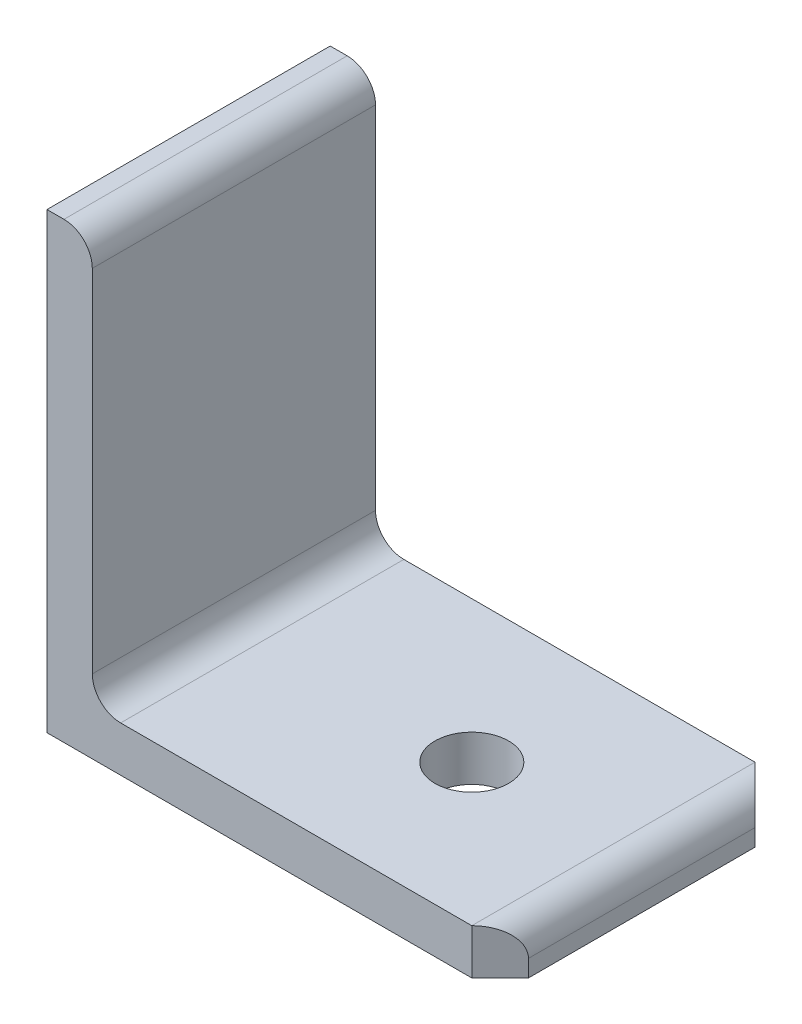
from build123d import *

# Parameters (mm, degrees)
EXTRUDE_1_DEPTH     = 50
SKETCH_2_R          = 6.5
CUT_EXTRUDE_1_DEPTH = 50
FILLET_1_R          = 5
FILLET_2_R          = 5
CHAMFER_1_SIZE      = 5
FILLET_3_R          = 5


with BuildPart() as part:
    # 草图1 → 凸台-拉伸1 (new body)
    with BuildSketch(Plane.XY):
        Polygon((0, 0), (0, -80), (80, -80), (80, -72), (8, -72), (8, 0), align=None)
    extrude(amount=EXTRUDE_1_DEPTH)

    # 草图2 → 切除-拉伸1 (cut)
    with BuildSketch(Plane(origin=(0, -72, 0), x_dir=(1, 0, 0), z_dir=(0, 1, 0))):
        with Locations(Location((50, -25, 0), (0, 0, 270))):
            Circle(SKETCH_2_R)
    extrude(amount=-CUT_EXTRUDE_1_DEPTH, mode=Mode.SUBTRACT)

    # 圆角1
    fillet_1_edges = [part.edges().sort_by_distance(p)[0] for p in [
        (8, -72, 25),
    ]]
    fillet(fillet_1_edges, radius=FILLET_1_R)

    # 圆角2
    fillet_2_edges = [part.edges().sort_by_distance(p)[0] for p in [
        (8, 0, 25),
    ]]
    fillet(fillet_2_edges, radius=FILLET_2_R)

    # 倒角1
    chamfer_1_edges = [part.edges().sort_by_distance(p)[0] for p in [
        (80, -76, 0),
        (80, -76, 50),
    ]]
    chamfer(chamfer_1_edges, length=CHAMFER_1_SIZE)

    # 圆角3
    fillet_3_edges = [part.edges().sort_by_distance(p)[0] for p in [
        (80, -72, 25),
    ]]
    fillet(fillet_3_edges, radius=FILLET_3_R)


solid = part.part
